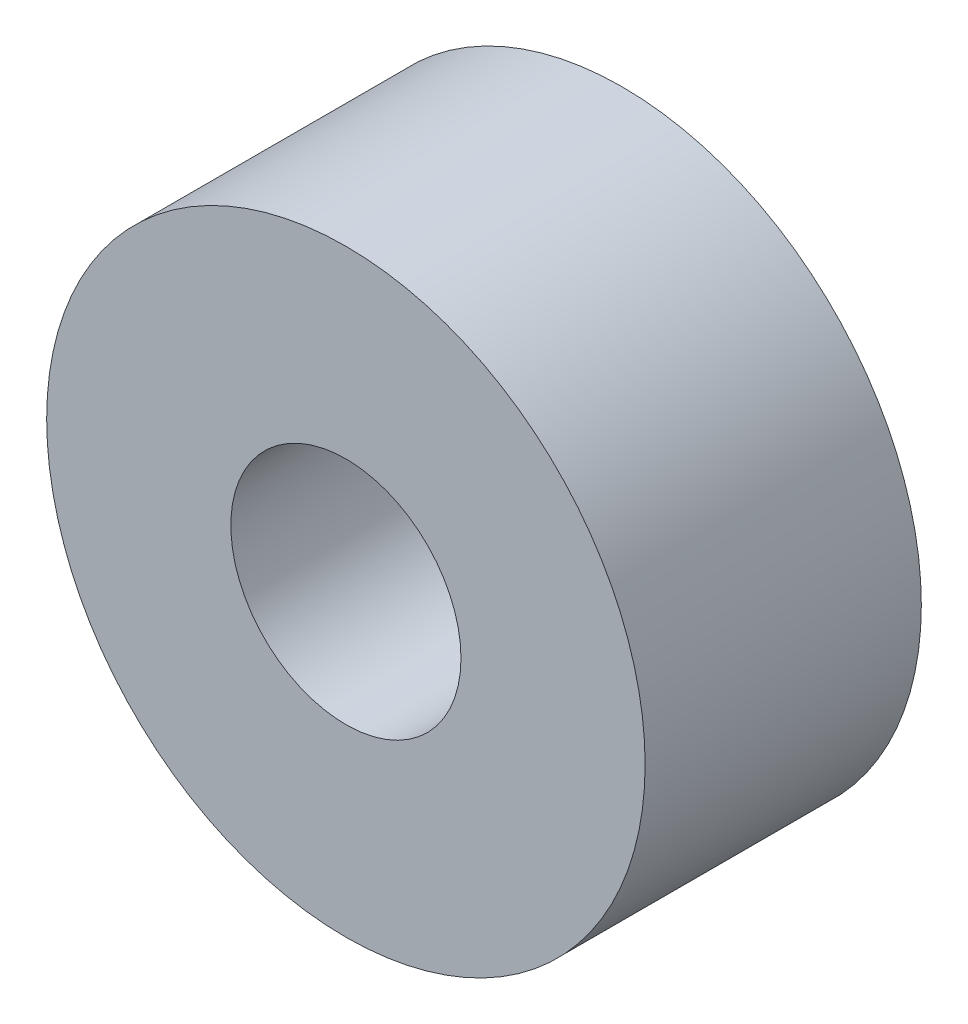
SolidWorks part; units mm, degrees
ref_plane "Front Plane" through (0, 0, 0) normal (0, 0, 1) x (1, 0, 0)
ref_plane "Top Plane" through (0, 0, 0) normal (0, 1, 0) x (1, 0, 0)
ref_plane "Right Plane" through (0, 0, 0) normal (1, 0, 0) x (0, 0, -1)
other "Configuration Table"
sketch "Sketch1" plane through (0, 0, -6) normal (0, 0, 1) x (1, 0, 0)
  circle A0 centre (0, 0) radius 6.5
  circle A1 centre (0, 0) radius 2.5
extrude "Boss-Extrude1" add sketch "Sketch1" along normal blind 6
